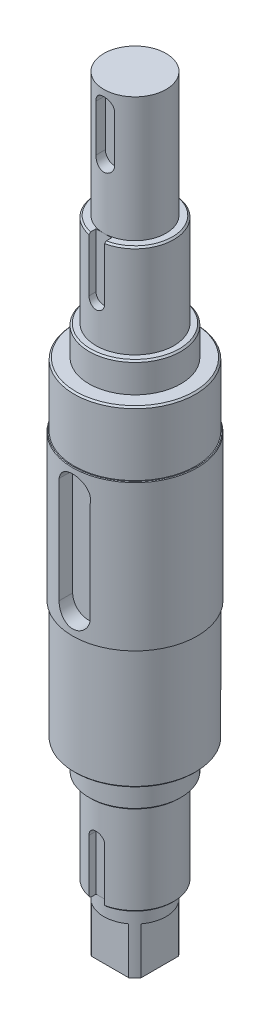
from build123d import *

# Parameters (mm, degrees)
EXTRUDE1_DEPTH       = 32
EXTRUDE1_DEPTH_BACK  = 15
SKETCH1_R            = 20
SKETCH_1_R           = 19.5
EXTRUDE_1_DEPTH      = 38.5
EXTRUDE2_START       = 20.5
SKETCH2_R            = 19.5
EXTRUDE2_DEPTH       = 20.5
CHAMFER1_SIZE        = 0.2
CUT_EXTRUDE1_DEPTH   = 5
SKETCH5_R            = 14.75
EXTRUDE3_DEPTH       = 9.5
SKETCH6_R            = 12.5
EXTRUDE4_DEPTH       = 30
EXTRUDE5_START       = 9.5
SKETCH7_R            = 14.75
EXTRUDE5_DEPTH       = 9.5
EXTRUDE6_START       = 30
SKETCH8_R            = 12.5
EXTRUDE6_DEPTH       = 30
CHAMFER2_SIZE        = 0.5
SKETCH9_R            = 10
EXTRUDE7_DEPTH       = 40
CUT_EXTRUDE2_DEPTH   = 4.5
BOSS_EXTRUDE1_START  = 20
SKETCH11_R           = 10
BOSS_EXTRUDE1_DEPTH  = 20
SKETCH12_OUTSIDE_W   = 92.29
SKETCH12_OUTSIDE_H   = 92.29
SKETCH12_OUTSIDE_W_2 = 16
SKETCH12_OUTSIDE_H_2 = 16
CUT_EXTRUDE3_DEPTH   = 15
CHAMFER3_SIZE        = 0.5
CUT_EXTRUDE4_DEPTH   = 10


with BuildPart() as part:
    # Sketch1 → Extrude1 (new, two sides: drawn at the far end of the back side and taken through both)
    with BuildSketch(Plane(origin=(0, 0, 0), x_dir=(1, 0, 0), z_dir=(0, 1, 0)).offset(-EXTRUDE1_DEPTH_BACK)):
        with Locations(Location((0, 0, 0), (0, 0, 270))):
            Circle(SKETCH1_R)
    extrude(amount=EXTRUDE1_DEPTH + EXTRUDE1_DEPTH_BACK)

    # 草图1 → 拉伸1 (add)
    with BuildSketch(Plane.XZ.offset(15)):
        with Locations(Location((0, 0, 0), (0, 0, 90))):
            Circle(SKETCH_1_R)
    extrude(amount=EXTRUDE_1_DEPTH)

    # Sketch2 → Extrude2 (add)
    with BuildSketch(Plane(origin=(0, 32, 0), x_dir=(1, 0, 0), z_dir=(0, 1, 0)).offset(EXTRUDE2_START)):
        with Locations(Location((0, 0, 0), (0, 0, 270))):
            Circle(SKETCH2_R)
    extrude(amount=-EXTRUDE2_DEPTH)

    # Chamfer1
    chamfer1_edges = [part.edges().sort_by_distance(p)[0] for p in [
        (0, 32, -20),
    ]]
    chamfer(chamfer1_edges, length=CHAMFER1_SIZE)

    # Sketch4 → Cut-Extrude1 (cut)
    with BuildSketch(Plane.XY.offset(20)):
        with BuildLine():
            Line((-5, 26), (-5, -8))
            ThreePointArc((-5, -8), (0, -13), (5, -8))
            Line((5, -8), (5, 24))
            ThreePointArc((5, 24), (1, 30), (-5, 26))
        make_face()
    extrude(amount=-CUT_EXTRUDE1_DEPTH, mode=Mode.SUBTRACT)

    # Sketch5 → Extrude3 (add)
    with BuildSketch(Plane(origin=(0, 52.5, 0), x_dir=(1, 0, 0), z_dir=(0, 1, 0))):
        with Locations(Location((0, 0, 0), (0, 0, 270))):
            Circle(SKETCH5_R)
    extrude(amount=EXTRUDE3_DEPTH)

    # Sketch6 → Extrude4 (add)
    with BuildSketch(Plane(origin=(0, 62, 0), x_dir=(1, 0, 0), z_dir=(0, 1, 0))):
        with Locations(Location((0, 0, 0), (0, 0, 270))):
            Circle(SKETCH6_R)
    extrude(amount=EXTRUDE4_DEPTH)

    # Sketch7 → Extrude5 (add)
    with BuildSketch(Plane.XZ.offset(53.5).offset(EXTRUDE5_START)):
        with Locations(Location((0, 0, 0), (0, 0, 90))):
            Circle(SKETCH7_R)
    extrude(amount=-EXTRUDE5_DEPTH)

    # Sketch8 → Extrude6 (add)
    with BuildSketch(Plane.XZ.offset(63).offset(EXTRUDE6_START)):
        with Locations(Location((0, 0, 0), (0, 0, 90))):
            Circle(SKETCH8_R)
    extrude(amount=-EXTRUDE6_DEPTH)

    # Chamfer2
    chamfer2_edges = [part.edges().sort_by_distance(p)[0] for p in [
        (0, 52.5, -19.5),
        (0, 62, -14.75),
        (0, 92, -12.5),
        (0, -63, -14.75),
        (0, -53.5, -19.5),
    ]]
    chamfer(chamfer2_edges, length=CHAMFER2_SIZE)

    # Sketch9 → Extrude7 (add)
    with BuildSketch(Plane(origin=(0, 92, 0), x_dir=(1, 0, 0), z_dir=(0, 1, 0))):
        with Locations(Location((0, 0, 0), (0, 0, 270))):
            Circle(SKETCH9_R)
    extrude(amount=EXTRUDE7_DEPTH)

    # Sketch10 → Cut-Extrude2 (cut)
    with BuildSketch(Plane.XY.offset(11)):
        with BuildLine():
            Line((-3, 127), (-3, 112))
            ThreePointArc((-3, 112), (0, 109), (3, 112))
            Line((3, 112), (3, 127))
            ThreePointArc((3, 127), (0, 130), (-3, 127))
        make_face()
    extrude(amount=-CUT_EXTRUDE2_DEPTH, mode=Mode.SUBTRACT)

    # Sketch11 → Boss-Extrude1 (add)
    with BuildSketch(Plane.XZ.offset(93).offset(BOSS_EXTRUDE1_START)):
        with Locations(Location((0, 0, 0), (0, 0, 90))):
            Circle(SKETCH11_R)
    extrude(amount=-BOSS_EXTRUDE1_DEPTH)

    # Sketch12 outside → Cut-Extrude3 (cut)
    with BuildSketch(Plane.XZ.offset(113)):
        Rectangle(SKETCH12_OUTSIDE_W, SKETCH12_OUTSIDE_H)
        Rectangle(SKETCH12_OUTSIDE_W_2, SKETCH12_OUTSIDE_H_2, mode=Mode.SUBTRACT)
    extrude(amount=-CUT_EXTRUDE3_DEPTH, mode=Mode.SUBTRACT)

    # Chamfer3
    chamfer3_edges = [part.edges().sort_by_distance(p)[0] for p in [
        (0, -93, -12.5),
    ]]
    chamfer(chamfer3_edges, length=CHAMFER3_SIZE)

    # Sketch13 → Cut-Extrude4 (cut)
    with BuildSketch(Plane.XY.offset(10)):
        with BuildLine():
            Line((2.5, 92), (2.5, 74.5))
            ThreePointArc((2.5, 74.5), (0, 72), (-2.5, 74.5))
            Line((-2.5, 74.5), (-2.5, 92))
            ThreePointArc((-2.5, 92), (0, 94.5), (2.5, 92))
        make_face()
        with BuildLine():
            Line((-2.5, -93), (-2.5, -75.5))
            ThreePointArc((-2.5, -75.5), (0, -73), (2.5, -75.5))
            Line((2.5, -75.5), (2.5, -93))
            ThreePointArc((2.5, -93), (0, -95.5), (-2.5, -93))
        make_face()
    extrude(amount=CUT_EXTRUDE4_DEPTH, mode=Mode.SUBTRACT)


solid = part.part
